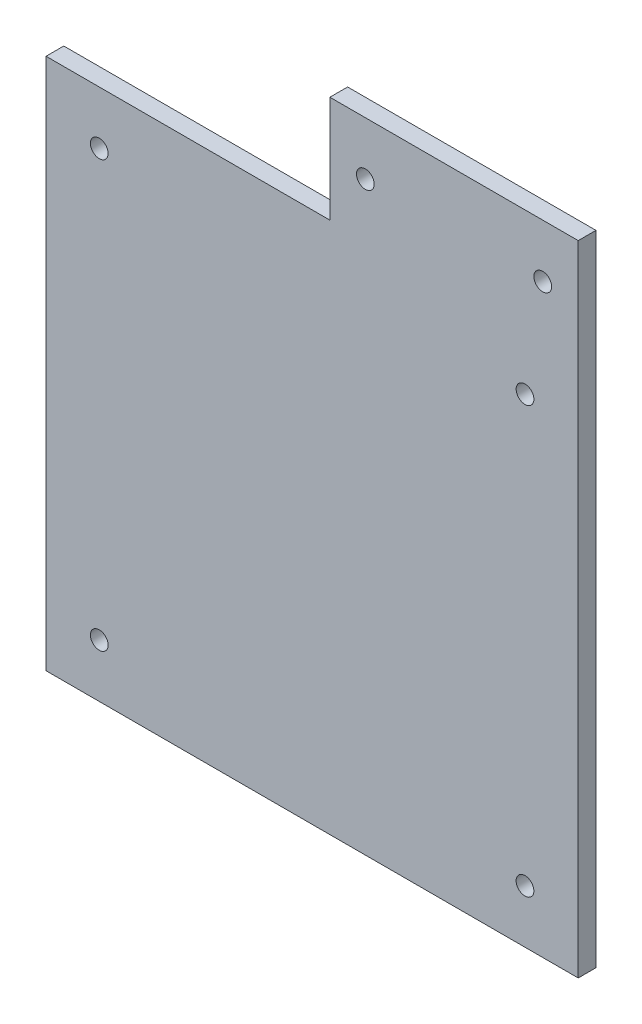
from build123d import *

# Parameters (mm, degrees)
SKETCH_1_R          = 5
EXTRUDE_1_DEPTH     = 10
SKETCH_3_W          = 10
SKETCH_3_H          = 60
EXTRUDE_2_DEPTH     = 40
CUT_EXTRUDE_2_DEPTH = 40


with BuildPart() as part:
    # 草图1 → 凸台-拉伸1 (new body)
    with BuildSketch(Plane.XY):
        Polygon((300, 360), (200, 360), (200, 300), (0, 300), (0, 0), (300, 0), (300, 300), align=None)
        with Locations((270, 30)):
            Circle(SKETCH_1_R, mode=Mode.SUBTRACT)
        with Locations((30, 30)):
            Circle(SKETCH_1_R, mode=Mode.SUBTRACT)
        with Locations((270, 270)):
            Circle(SKETCH_1_R, mode=Mode.SUBTRACT)
        with Locations((30, 270)):
            Circle(SKETCH_1_R, mode=Mode.SUBTRACT)
    extrude(amount=EXTRUDE_1_DEPTH)

    # 草图3 → 凸台-拉伸2 (add)
    with BuildSketch(Plane.ZY.offset(-200)):
        with Locations((5, 330)):
            Rectangle(SKETCH_3_W, SKETCH_3_H)
    extrude(amount=EXTRUDE_2_DEPTH)

    # 草图4 → 切除-拉伸2 (cut)
    with BuildSketch(Plane.XY.offset(10)):
        with BuildLine():
            ThreePointArc((175, 330), (180, 325), (185, 330))
            Line((185, 330), (175, 330))
        make_face()
        with BuildLine():
            Line((175, 330), (185, 330))
            ThreePointArc((185, 330), (180, 335), (175, 330))
        make_face()
        with BuildLine():
            ThreePointArc((285, 330), (280, 335), (275, 330))
            Line((275, 330), (280, 330))
            Line((280, 330), (285, 330))
        make_face()
        with BuildLine():
            Line((280, 330), (275, 330))
            ThreePointArc((275, 330), (280, 325), (285, 330))
            Line((285, 330), (280, 330))
        make_face()
    extrude(amount=-CUT_EXTRUDE_2_DEPTH, mode=Mode.SUBTRACT)


solid = part.part
